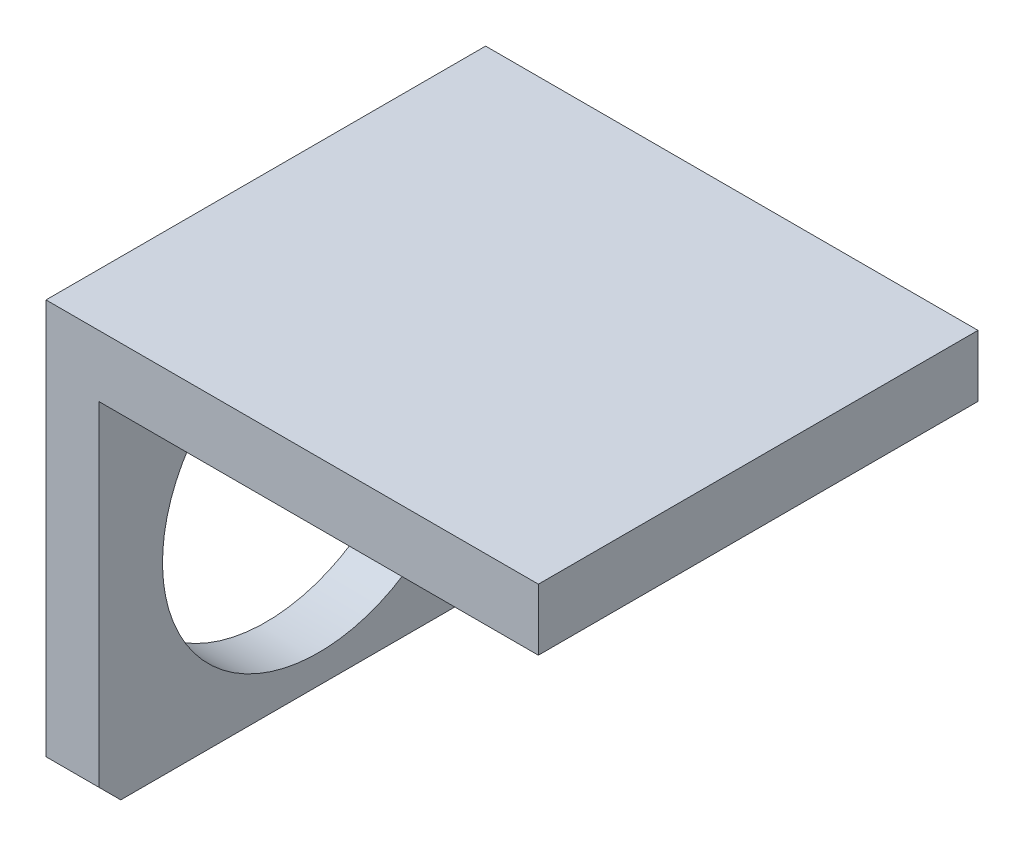
SolidWorks part; units mm, degrees
ref_plane "前视基准面" through (0, 0, 0) normal (0, 0, 1) x (1, 0, 0)
ref_plane "上视基准面" through (0, 0, 0) normal (0, 1, 0) x (1, 0, 0)
ref_plane "右视基准面" through (0, 0, 0) normal (1, 0, 0) x (0, 0, -1)
sketch "草图1" plane through (0, 0, 0) normal (0, 0, 1) x (1, 0, 0)
  line L0 (0, 0) -> (0, 95)
  line L4 (12, 95) -> (12, 0)
  line L5 (12, 0) -> (0, 0)
  line L6 (12, 95) -> (0, 95)
  dimension "D1" = 12
  dimension "D4" = 95
extrude "凸台-拉伸1" add sketch "草图1" along normal mid plane 100
sketch "草图2" plane through (12, 0, 0) normal (1, 0, 0) x (0, 0, -1)
  line L0 (-50, 0) -> (50, 0) construction
  circle A0 centre (0, 42) radius 35.5
  dimension "D2" = 71
  dimension "D1" = 42
extrude "切除-拉伸1" cut sketch "草图2" against normal up to next
sketch "草图3" plane through (12, 0, 0) normal (1, 0, 0) x (0, 0, -1)
  line L0 (50, 0) -> (50, 95) construction
  line L1 (-50, 95) -> (50, 95)
  line L2 (-50, 95) -> (-50, 81)
  line L3 (-50, 81) -> (50, 81)
  line L4 (50, 95) -> (50, 81)
  dimension "D1" = 14
extrude "凸台-拉伸2" add sketch "草图3" along normal blind 100
chamfer "倒角1" distance 5 angle 45 2 edges at (6, 0, 50) (6, 0, -50)
